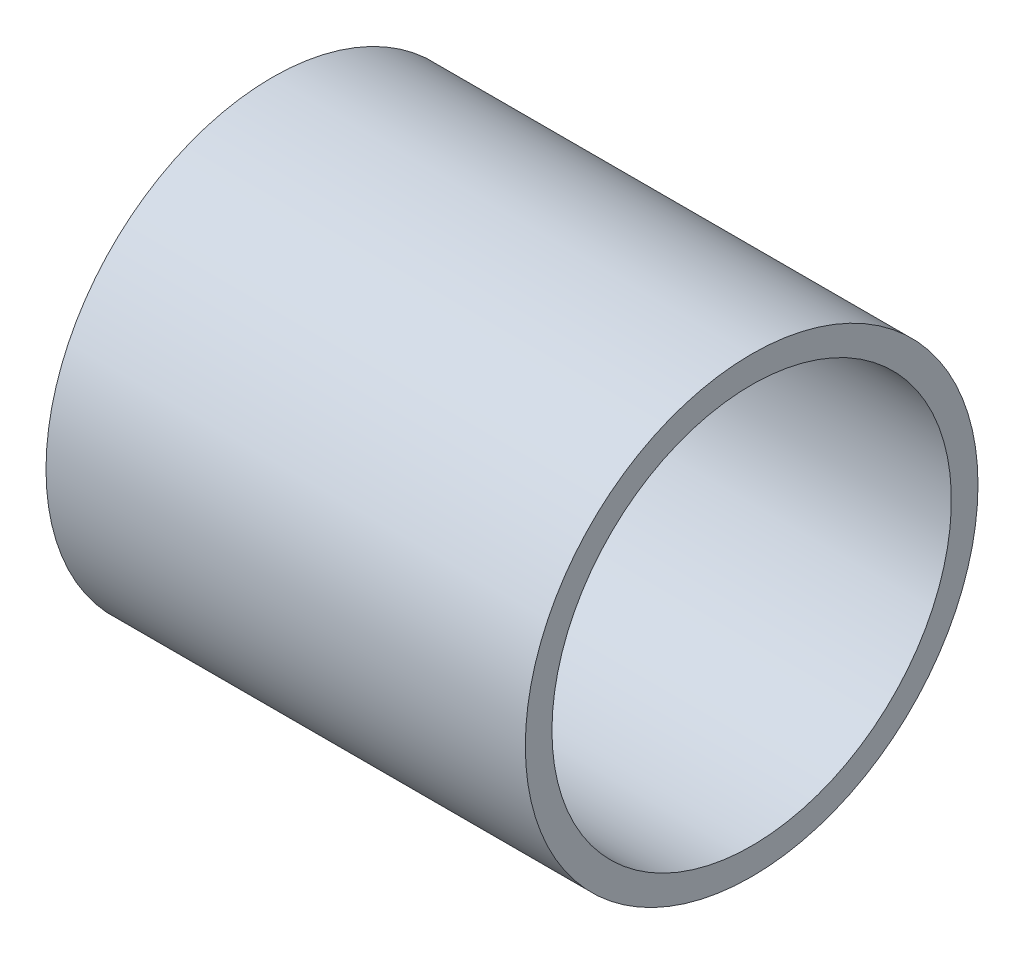
SolidWorks part; units mm, degrees
ref_plane "Front Plane" through (0, 0, 0) normal (0, 0, 1) x (1, 0, 0)
ref_plane "Top Plane" through (0, 0, 0) normal (0, 1, 0) x (1, 0, 0)
ref_plane "Right Plane" through (0, 0, 0) normal (1, 0, 0) x (0, 0, -1)
other "Configuration Table"
sketch "Sketch1" plane through (0, 0, 0) normal (1, 0, 0) x (0, 0, -1)
  circle A0 centre (0, 0) radius 85
  circle A1 centre (0, 0) radius 75
  dimension "D1" = 170
  dimension "D2" = 150
extrude "Boss-Extrude1" add sketch "Sketch1" along normal blind 180
